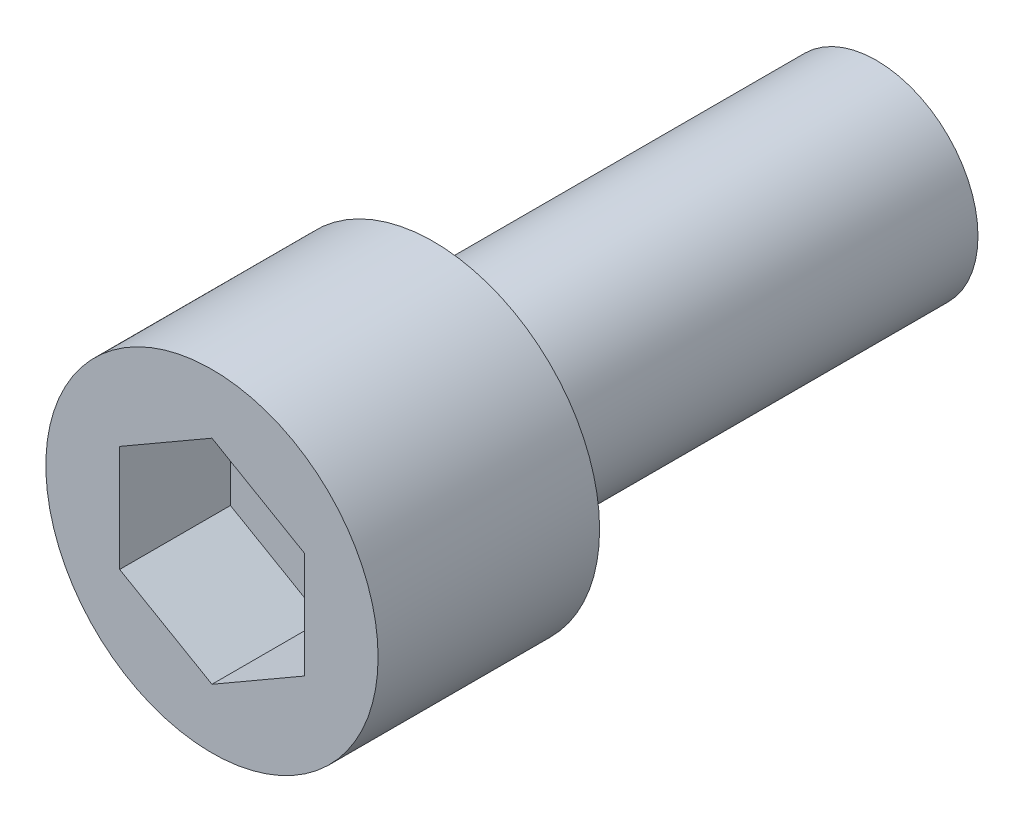
SolidWorks part; units mm, degrees
ref_plane "Front Plane" through (0, 0, 0) normal (0, 0, 1) x (1, 0, 0)
ref_plane "Top Plane" through (0, 0, 0) normal (0, 1, 0) x (1, 0, 0)
ref_plane "Right Plane" through (0, 0, 0) normal (1, 0, 0) x (0, 0, -1)
sketch "Sketch1" plane through (0, 0, 0) normal (0, 0, 1) x (1, 0, 0)
  circle A0 centre (0, 0) radius 5.5
extrude "Boss-Extrude1" add sketch "Sketch1" along normal blind 24
cosmetic thread "Cosmetic Thread1" parameters "D1"=18, "D2"=10
sketch "Sketch2" plane through (0, 0, 24) normal (0, 0, 1) x (1, 0, 0)
  circle A0 centre (0, 0) radius 9
extrude "Boss-Extrude2" add sketch "Sketch2" along normal blind 12
sketch "Sketch3" plane through (0, 0, 36) normal (0, 0, 1) x (1, 0, 0)
  line L1 (0, 5.7735) -> (-5, 2.8868)
  line L2 (-5, 2.8868) -> (-5, -2.8868)
  line L3 (-5, -2.8868) -> (0, -5.7735)
  line L4 (0, -5.7735) -> (5, -2.8868)
  line L5 (5, -2.8868) -> (5, 2.8868)
  line L6 (5, 2.8868) -> (0, 5.7735)
  circle A0 centre (0, 0) radius 5 construction
  dimension "D1" = 10
extrude "Cut-Extrude1" cut sketch "Sketch3" against normal blind 6 contours L1 L2 L3 L4 L5 L6
